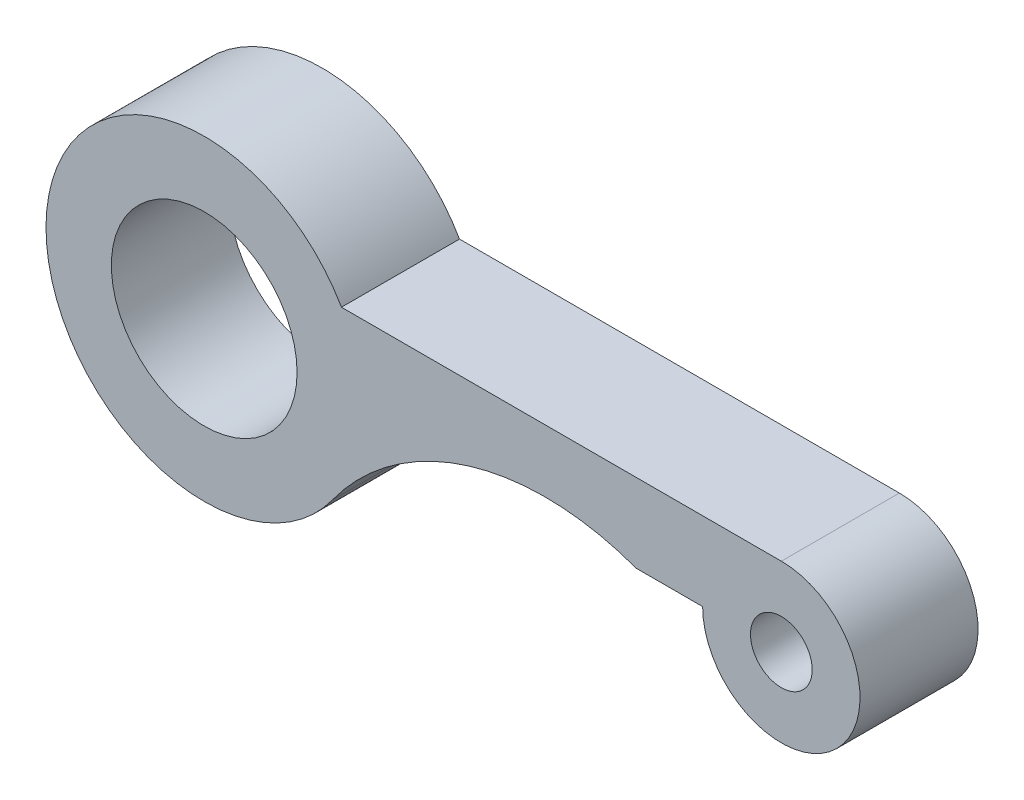
from build123d import *

# Parameters (mm, degrees)
SKETCH_1_R      = 3.54
SKETCH_1_R_2    = 1.176
EXTRUDE_1_DEPTH = 4.5


with BuildPart() as part:
    # 草图1 → 凸台-拉伸1 (new body)
    with BuildSketch(Plane.XY):
        with BuildLine():
            Line((22, 3), (5.232070686, 3))
            ThreePointArc((5.232070686, 3), (-6.022909015, 0.314850207), (4.890755195, -3.529175156))
            ThreePointArc((4.890755195, -3.529175156), (10.083161164, 0.184396071), (16.464202545, 0))
            Line((16.464202545, 0), (19, 0))
            ThreePointArc((19, 0), (24.121320344, -2.121320344), (22, 3))
        make_face()
        Circle(SKETCH_1_R, mode=Mode.SUBTRACT)
        with Locations((22, 0)):
            Circle(SKETCH_1_R_2, mode=Mode.SUBTRACT)
    extrude(amount=EXTRUDE_1_DEPTH)


solid = part.part
